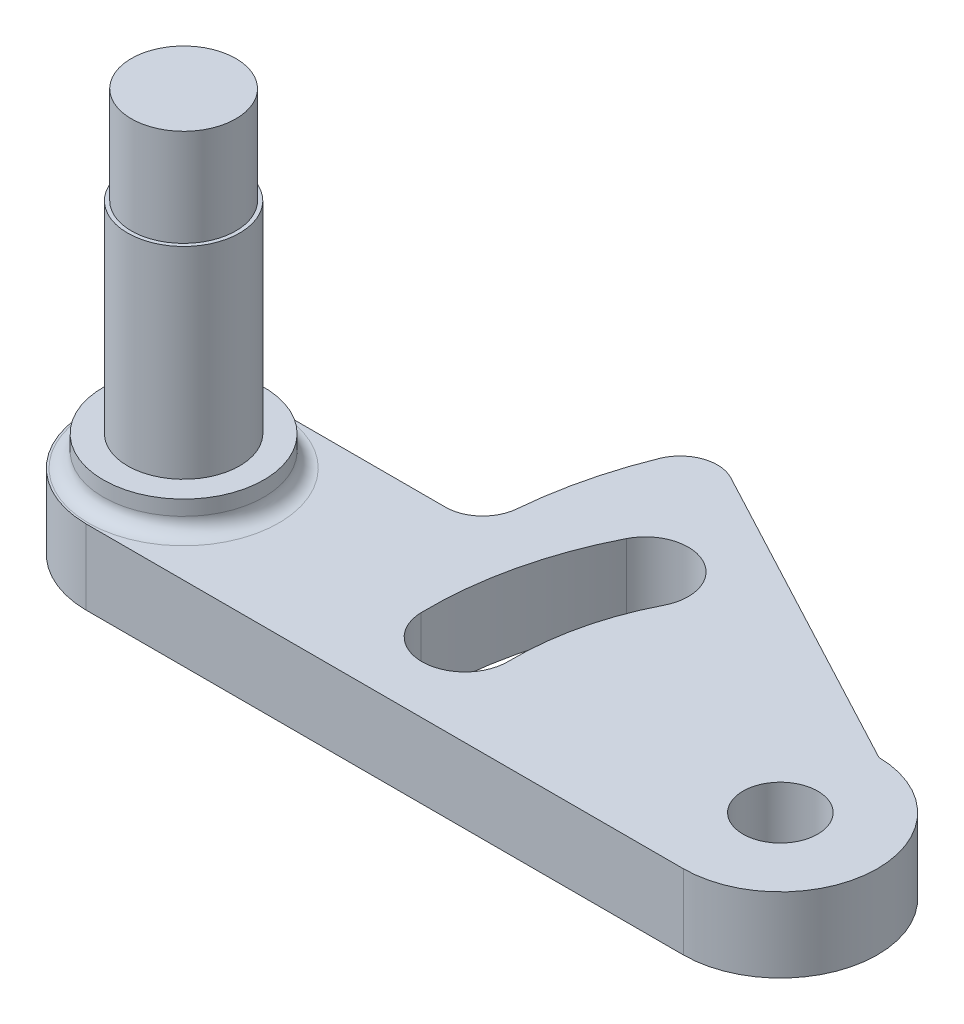
SolidWorks part; units mm, degrees
ref_plane "前视基准面" through (0, 0, 0) normal (0, 0, 1) x (1, 0, 0)
ref_plane "上视基准面" through (0, 0, 0) normal (0, 1, 0) x (1, 0, 0)
ref_plane "右视基准面" through (0, 0, 0) normal (1, 0, 0) x (0, 0, -1)
sketch "草图1" plane through (0, 0, 0) normal (0, 1, 0) x (1, 0, 0)
  line L0 (0, 0) -> (80, 0)
  line L1 (80.1889, 25.9986) -> (33.172, 50.998)
  line L2 (0.1889, 26) -> (26.9389, 26)
  arc A0 (0.1889, 26) -> (0, 0) centre (0.0945, 13) ccw
  arc A1 (80, 0) -> (80.1889, 25.9986) centre (80, 13) ccw
  arc A2 (33.172, 50.998) -> (26.9389, 26) centre (80.1889, 25.9986) ccw
  circle A3 centre (80, 13) radius 5
  arc A5 (48.1622, 29.2609) -> (44.2558, 12.3539) centre (80, 13) ccw
  arc A6 (37.9207, 34.4917) -> (32.7577, 12.1461) centre (80, 13) ccw
  arc A7 (48.1622, 29.2609) -> (37.9207, 34.4917) centre (43.0414, 31.8763) ccw
  arc A8 (32.7577, 12.1461) -> (44.2558, 12.3539) centre (38.5068, 12.25) ccw
  dimension "D6" = 106.5
  dimension "D5" = 13
  dimension "D7" = 10
  dimension "D8" = 71.5
  dimension "D9" = 94.5
  dimension "D10" = 11.5
  dimension "D11" = 11.5
  dimension "D14" = 5.8763
  dimension "D1" = 26
  dimension "D2" = 80
  dimension "D3" = 80
  dimension "D4" = 28
  dimension "D12" = 12.25
  dimension "D13" = 12.25
extrude "凸台-拉伸1" add sketch "草图1" along normal blind 10
fillet "圆角2" radius 5 2 edges at (26.9389, 5, -26) (33.172, 5, -50.998)
sketch "草图2" plane through (0, 10, 0) normal (0, 1, 0) x (1, 0, 0)
  circle A0 centre (0.0945, 13) radius 10.75
  dimension "D1" = 21.5
extrude "凸台-拉伸2" add sketch "草图2" along normal blind 4
fillet "圆角3" radius 2 1 edges at (0.0945, 10, -2.25)
sketch "草图3" plane through (0, 14, 0) normal (0, 1, 0) x (1, 0, 0)
  circle A0 centre (0.0945, 13) radius 7.5
  dimension "D1" = 15
extrude "凸台-拉伸3" add sketch "草图3" along normal blind 27
sketch "草图5" plane through (0, 41, 0) normal (0, 1, 0) x (1, 0, 0)
  circle A0 centre (0.0945, 13) radius 7
  dimension "D1" = 14
extrude "凸台-拉伸4" add sketch "草图5" along normal blind 13 contours A0
cosmetic thread "装饰螺纹线1" parameters "D2"=8.566
